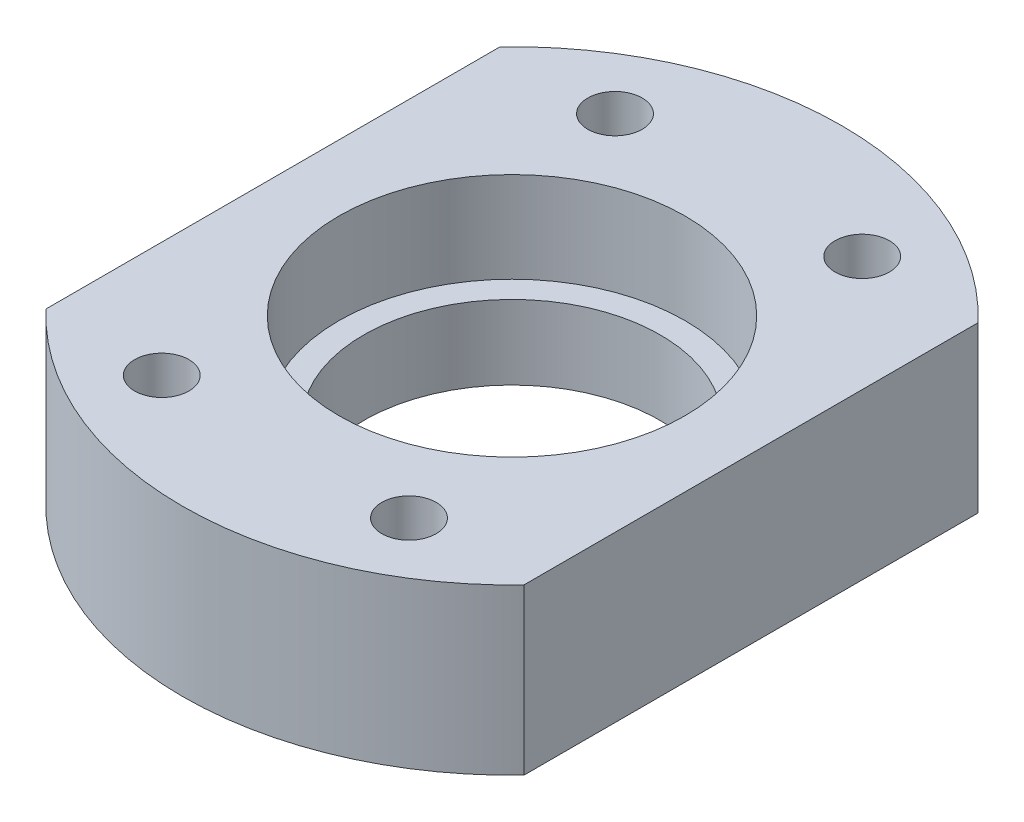
SolidWorks part; units mm, degrees
ref_plane "Front Plane" through (0, 0, 0) normal (0, 0, 1) x (1, 0, 0)
ref_plane "Top Plane" through (0, 0, 0) normal (0, 1, 0) x (1, 0, 0)
ref_plane "Right Plane" through (0, 0, 0) normal (1, 0, 0) x (0, 0, -1)
other "Configuration Table"
sketch "Sketch1" plane through (0, 0, 0) normal (0, 1, 0) x (1, 0, 0)
  circle A0 centre (0, 0) radius 40
  dimension "D1" = 80
extrude "Boss-Extrude1" add sketch "Sketch1" along normal blind 20
sketch "Sketch2" plane through (0, 20, 0) normal (0, 1, 0) x (1, 0, 0)
  circle A0 centre (0, 0) radius 21
  dimension "D1" = 42
extrude "Cut-Extrude1" cut sketch "Sketch2" against normal blind 11
sketch "Sketch3" plane through (0, 9, 0) normal (0, 1, 0) x (1, 0, 0)
  circle A0 centre (0, 0) radius 18
  dimension "D1" = 36
extrude "Cut-Extrude2" cut sketch "Sketch3" against normal blind 11
sketch "Sketch8" plane through (0, 0, 0) normal (0, -1, 0) x (1, 0, 0)
  line L2 (-29, -27.55) -> (-29, 27.55)
  line L4 (29, -27.55) -> (29, 27.55)
  line L5 (-29, -41.454) -> (29, 41.454) construction
  line L6 (-29, 41.454) -> (29, -41.454) construction
  circle A0 centre (0, 0) radius 40 construction
  arc A1 (-22.9291, -32.7759) -> (22.9291, -32.7759) centre (0, 0) ccw
  arc A2 (29, -27.55) -> (29, 27.55) centre (0, 0) ccw
  arc A3 (-29, 27.55) -> (-29, -27.55) centre (0, 0) ccw
  point P0 (0, 0)
  circle M10 centre (0, 0) radius 40
  dimension "D1" = 58
  dimension "D2" = 29
  dimension "D3" = 29
extrude "Cut-Extrude3" cut sketch "Sketch8" against normal through all contours L4 M10 | L2 M10
sketch "Sketch9" plane through (0, 0, 0) normal (0, -1, 0) x (1, 0, 0)
  circle A0 centre (0, 0) radius 27.5 construction
  dimension "D1" = 55
sketch "Sketch11" plane through (0, 0, 0) normal (0, -1, 0) x (1, 0, 0)
  line L0 (0, 0) -> (0, 27.5) construction
  line L1 (-15, 27.5) -> (15, 27.5) construction
  circle A0 centre (0, 0) radius 27.5 construction
  circle A1 centre (0, 0) radius 31.3249 construction
  point P8 (0, 27.5)
  dimension "D1" = 30
hole_wizard "M6 Clearance Hole2" positions "Sketch12" profile "Sketch13" hole size "M6" standard "GB" end condition through all
sketch "Sketch12" plane through (0, 0, 0) normal (0, -1, 0) x (-1, 0, 0)
  circle A0 centre (0, 0) radius 31.3249 construction
  point P0 (-15, -27.5)
  point P3 (15, -27.5)
  point P6 (15, 27.5)
  point P10 (-15, 27.5)
  dimension "D1" = 30
  dimension "D2" = 27.5
sketch "Sketch13" plane through (15, 0, 27.5) normal (1, 0, 0) x (0, 0, -1)
  line L0 (0, 0) -> (0, 20)
  line L1 (0, 20) -> (3.3, 20)
  line L2 (3.3, 20) -> (3.3, 0.025)
  line L3 (3.3, 0.025) -> (3.325, 0)
  line L5 (3.325, 0) -> (0, 0)
  line L6 (-3.3, 0.025) -> (-3.325, 0) construction
  line L11 (0, -6.35) -> (0, 107.95) construction
  dimension "通孔孔直径" = 6.6
  dimension "通孔孔深度" = 20
  dimension "近端锥形沉头孔直径" = 6.65
  dimension "近端锥形沉头孔角度" = 90
